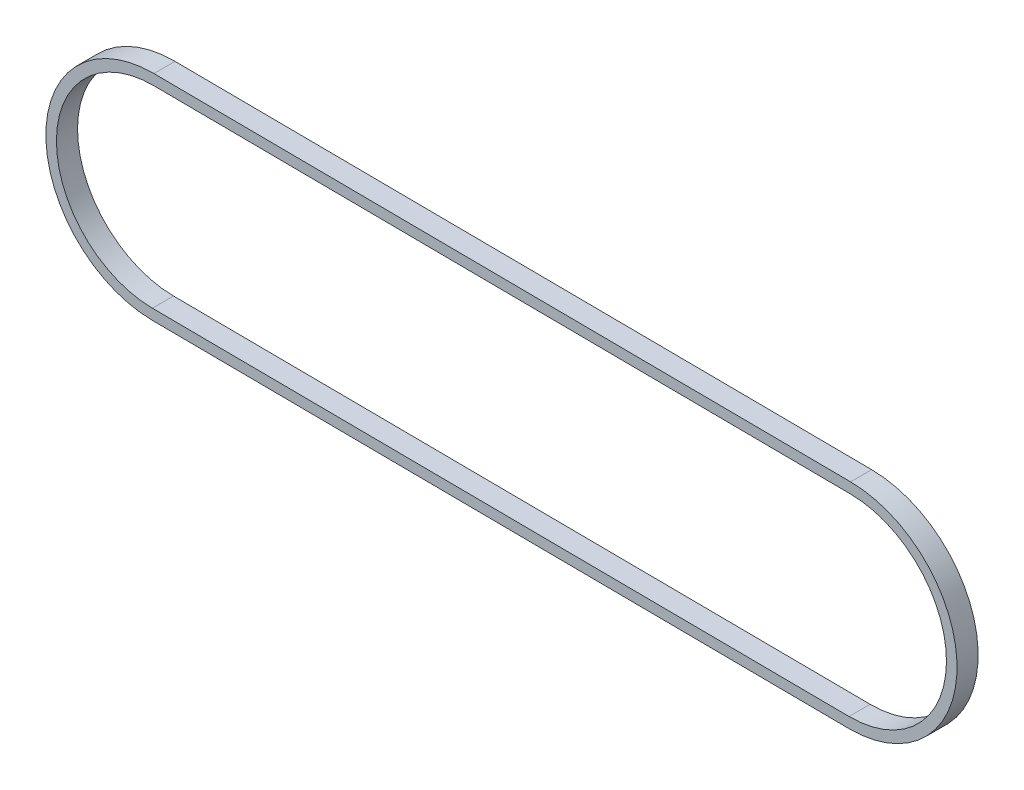
from build123d import *

# Parameters (mm, degrees)
EXTRUDE_1_DEPTH = 10


with BuildPart() as part:
    # 草图2 → 拉伸-薄壁1 (new, symmetric)
    with BuildSketch(Plane.XY):
        with BuildLine():
            Line((659.230135728, -106.622083889), (-0.769864272, -101.622083889))
            ThreePointArc((-0.769864272, -101.622083889), (-101.622083889, 0.769864272), (0.769864272, 101.622083889))
            Line((0.769864272, 101.622083889), (660.769864272, 96.622083889))
            ThreePointArc((660.769864272, 96.622083889), (761.622083889, -5.769864272), (659.230135728, -106.622083889))
        make_face()
        with BuildLine():
            Line((659.30589113, -96.622370837), (-0.69410887, -91.622370837))
            ThreePointArc((-0.69410887, -91.622370837), (-91.622370837, 0.69410887), (0.69410887, 91.622370837))
            Line((0.69410887, 91.622370837), (660.69410887, 86.622370837))
            ThreePointArc((660.69410887, 86.622370837), (751.622370837, -5.69410887), (659.30589113, -96.622370837))
        make_face(mode=Mode.SUBTRACT)
    extrude(amount=EXTRUDE_1_DEPTH, both=True)


solid = part.part
